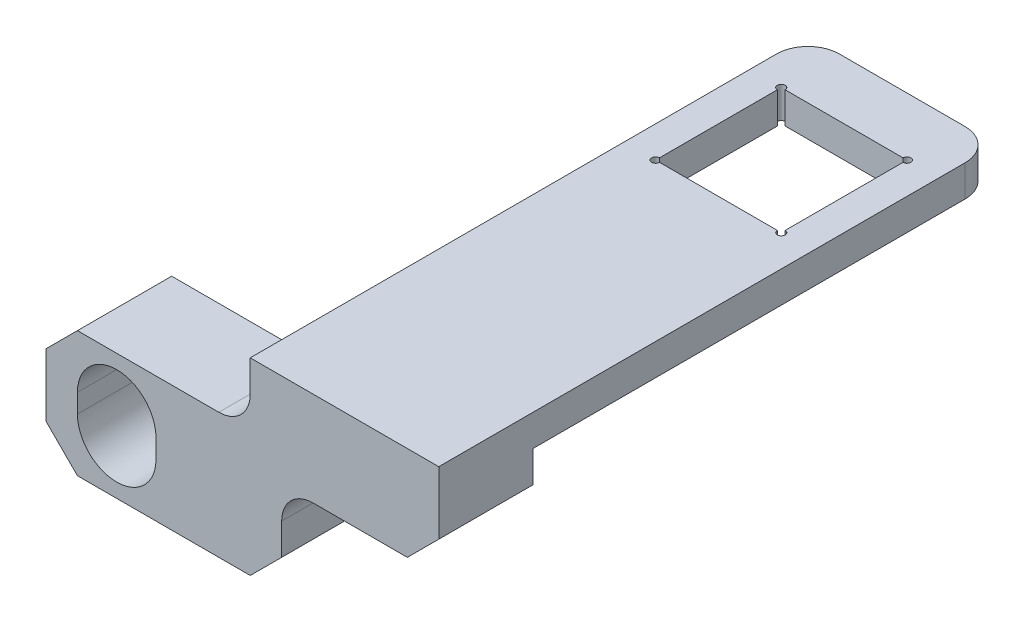
from build123d import *

# Parameters (mm, degrees)
SKETCH1_W             = 12
SKETCH1_H             = 43.5
BOSS_EXTRUDE1_DEPTH   = 2
M3_TAPPED_HOLE1_D     = 2.5
M3_TAPPED_HOLE1_DEPTH = 7.5
M3_TAPPED_HOLE1_TIP   = 0.751075774
SKETCH6_W             = 25
SKETCH6_H             = 12
BOSS_EXTRUDE2_DEPTH   = 14
SKETCH7_W             = 25
SKETCH7_H             = 8
CUT_EXTRUDE4_DEPTH    = 32.273990791
SKETCH8_R             = 2.5
CUT_EXTRUDE5_DEPTH    = 15
SKETCH9_W             = 13
SKETCH9_H             = 4
SKETCH9_W_2           = 10
SKETCH9_H_2           = 6
CUT_EXTRUDE6_DEPTH    = 18
CHAMFER2_SIZE         = 2
FILLET1_R             = 2
FILLET2_R             = 2
SKETCH3_W             = 8
SKETCH3_H             = 8
CUT_EXTRUDE2_DEPTH    = 10
SKETCH10_R            = 0.25
CUT_EXTRUDE7_DEPTH    = 10
CUT_EXTRUDE8_DEPTH    = 10


with BuildPart() as part:
    # Sketch1 → Boss-Extrude1 (new body)
    with BuildSketch(Plane(origin=(0, 0, 0), x_dir=(1, 0, 0), z_dir=(0, 1, 0))):
        Rectangle(SKETCH1_W, SKETCH1_H)
    extrude(amount=BOSS_EXTRUDE1_DEPTH)

    # M3 Tapped Hole1
    with Locations(Plane(origin=(0, 2, 17.75), x_dir=(0, 0, 1), z_dir=(0, 1, 0))):
        with Locations((0, 0)):
            Hole(M3_TAPPED_HOLE1_D / 2, depth=M3_TAPPED_HOLE1_DEPTH)
            with Locations((0, 0, -(M3_TAPPED_HOLE1_DEPTH + M3_TAPPED_HOLE1_TIP / 2))):  # 118° drill point
                Cone(0, M3_TAPPED_HOLE1_D / 2, M3_TAPPED_HOLE1_TIP, mode=Mode.SUBTRACT)

    # Sketch6 → Boss-Extrude2 (add)
    with BuildSketch(Plane.XY.offset(21.75)):
        with Locations((-6.5, -4)):
            Rectangle(SKETCH6_W, SKETCH6_H)
    extrude(amount=-BOSS_EXTRUDE2_DEPTH)

    # Sketch7 → Cut-Extrude4 (cut, through all)
    with BuildSketch(Plane(origin=(0, 2, 0), x_dir=(1, 0, 0), z_dir=(0, 1, 0))):
        with Locations((-6.5, -17.75)):
            Rectangle(SKETCH7_W, SKETCH7_H)
    extrude(amount=-CUT_EXTRUDE4_DEPTH, mode=Mode.SUBTRACT)

    # Sketch8 → Cut-Extrude5 (cut)
    with BuildSketch(Plane.XY.offset(13.75)):
        with Locations((-14.5, -6)):
            Circle(SKETCH8_R)
    extrude(amount=-CUT_EXTRUDE5_DEPTH, mode=Mode.SUBTRACT)

    # Sketch9 → Cut-Extrude6 (cut)
    with BuildSketch(Plane.XY.offset(13.75)):
        with Locations((-12.5, 0)):
            Rectangle(SKETCH9_W, SKETCH9_H)
        with Locations((1, -7)):
            Rectangle(SKETCH9_W_2, SKETCH9_H_2)
    extrude(amount=-CUT_EXTRUDE6_DEPTH, mode=Mode.SUBTRACT)

    # Chamfer2
    chamfer2_edges = [part.edges().sort_by_distance(p)[0] for p in [
        (-19, -10, 10.75),
        (-19, -2, 10.75),
        (6, -4, 10.75),
        (-4, -10, 10.75),
    ]]
    chamfer(chamfer2_edges, length=CHAMFER2_SIZE)

    # Fillet1
    fillet1_edges = [part.edges().sort_by_distance(p)[0] for p in [
        (-4, -4, 10.75),
        (-6, -2, 10.75),
    ]]
    fillet(fillet1_edges, radius=FILLET1_R)

    # Fillet2
    fillet2_edges = [part.edges().sort_by_distance(p)[0] for p in [
        (-6, 1, -21.75),
        (6, 1, -21.75),
    ]]
    fillet(fillet2_edges, radius=FILLET2_R)

    # Sketch3 → Cut-Extrude2 (cut)
    with BuildSketch(Plane(origin=(0, 2, 0), x_dir=(1, 0, 0), z_dir=(0, 1, 0))):
        with Locations((0, 14.05)):
            Rectangle(SKETCH3_W, SKETCH3_H)
    extrude(amount=-CUT_EXTRUDE2_DEPTH, mode=Mode.SUBTRACT)

    # Sketch10 → Cut-Extrude7 (cut)
    with BuildSketch(Plane(origin=(0, 2, 0), x_dir=(1, 0, 0), z_dir=(0, 1, 0))):
        with Locations((-4, 10.05)):
            Circle(SKETCH10_R)
        with Locations((4, 10.05)):
            Circle(SKETCH10_R)
        with Locations((-4, 18.05)):
            Circle(SKETCH10_R)
        with Locations((4, 18.05)):
            Circle(SKETCH10_R)
    extrude(amount=-CUT_EXTRUDE7_DEPTH, mode=Mode.SUBTRACT)

    # Sketch11 → Cut-Extrude8 (cut)
    with BuildSketch(Plane.XY.offset(13.75)):
        with BuildLine():
            Line((-12, -5.4), (-12, -6.6))
            ThreePointArc((-12, -6.6), (-14.5, -9.1), (-17, -6.6))
            Line((-17, -6.6), (-17, -5.4))
            ThreePointArc((-17, -5.4), (-14.5, -2.9), (-12, -5.4))
        make_face()
    extrude(amount=-CUT_EXTRUDE8_DEPTH, mode=Mode.SUBTRACT)


solid = part.part
